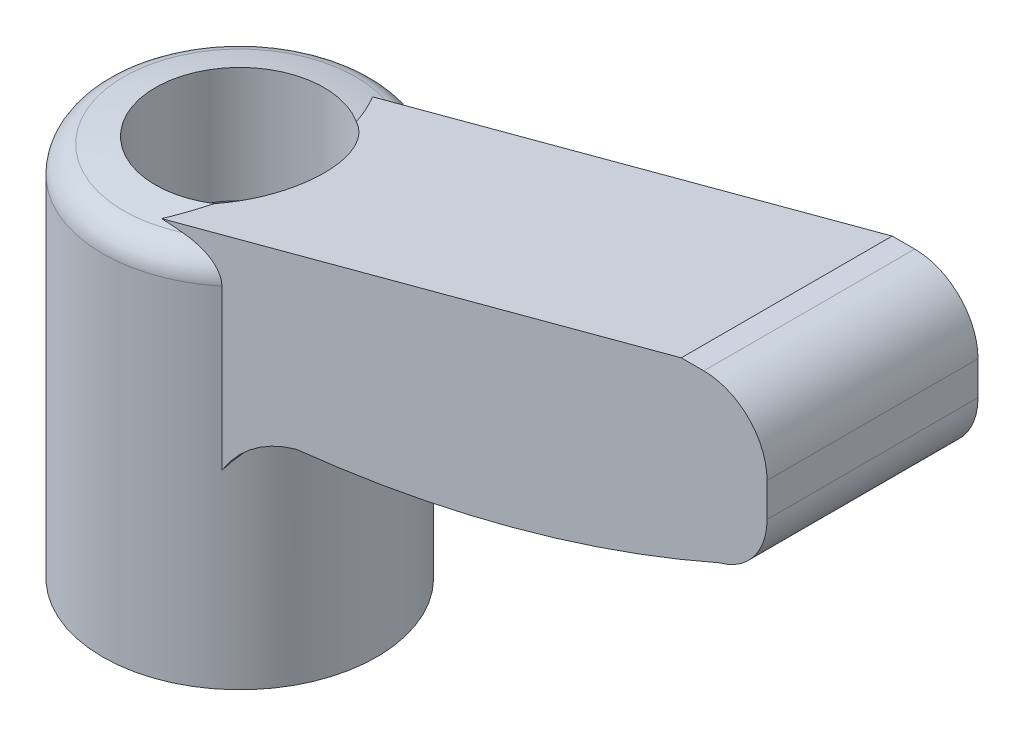
from build123d import *

# Parameters (mm, degrees)
EXTRUDE_1_DEPTH      = 5
EXTRUDE_1_DEPTH_BACK = 5


with BuildPart() as part:
    # 草图2 → 旋转1 (revolve)
    with BuildSketch(Plane.XY, mode=Mode.PRIVATE) as revolve_1_sk:
        with BuildLine():
            Line((6.5, 21.057334971), (6.5, 4.5))
            Line((6.5, 4.5), (5.633974596, 4))
            Line((5.633974596, 4), (0, 4))
            Line((0, 4), (0, 22.97165153))
            ThreePointArc((0, 22.97165153), (2.770599147, 22.808562355), (5.502930419, 22.321547438))
            ThreePointArc((5.502930419, 22.321547438), (6.220737367, 21.862378589), (6.5, 21.057334971))
        make_face()
    revolve(revolve_1_sk.sketch.rotate(Axis((0, 4, 0), (0, 1, 0)), 270), axis=Axis((0, 4, 0), (0, 1, 0)))

    # 草图1 → 凸台-拉伸1 (add, two sides: drawn at the far end of the back side and taken through both)
    with BuildSketch(Plane.XY.offset(-EXTRUDE_1_DEPTH_BACK)):
        with BuildLine():
            Line((-3.333333333, 5.5), (3.25, 5.5))
            Line((3.25, 5.5), (3.25, 10.326555972))
            ThreePointArc((3.25, 10.326555972), (4.489879958, 13.979124546), (7.697085729, 16.12211093))
            ThreePointArc((7.697085729, 16.12211093), (17.943826668, 18.039495945), (27.776457135, 21.502362282))
            ThreePointArc((27.776457135, 21.502362282), (29.380060021, 22.573855474), (30, 24.400139761))
            Line((30, 24.400139761), (30, 26))
            ThreePointArc((30, 26), (29.121320344, 28.121320344), (27, 29))
            Line((27, 29), (25.932943889, 29))
            Line((25.932943889, 29), (-3.333333333, 21.158124653))
            Line((-3.333333333, 21.158124653), (-3.333333333, 5.5))
        make_face()
    extrude(amount=EXTRUDE_1_DEPTH + EXTRUDE_1_DEPTH_BACK)

    # 草图3 → 切除-旋转1 (revolve, cut)
    with BuildSketch(Plane.XY, mode=Mode.PRIVATE) as cut_revolve_1_sk:
        Polygon((0, 28.156296), (4, 28.156296), (4, 17.156296), (5, 17.156296), (5, -2.643704), (0, -2.643704), align=None)
    revolve(cut_revolve_1_sk.sketch.rotate(Axis((0, -2.643704, 0), (0, 1, 0)), 270), axis=Axis((0, -2.643704, 0), (0, 1, 0)), mode=Mode.SUBTRACT)


solid = part.part
